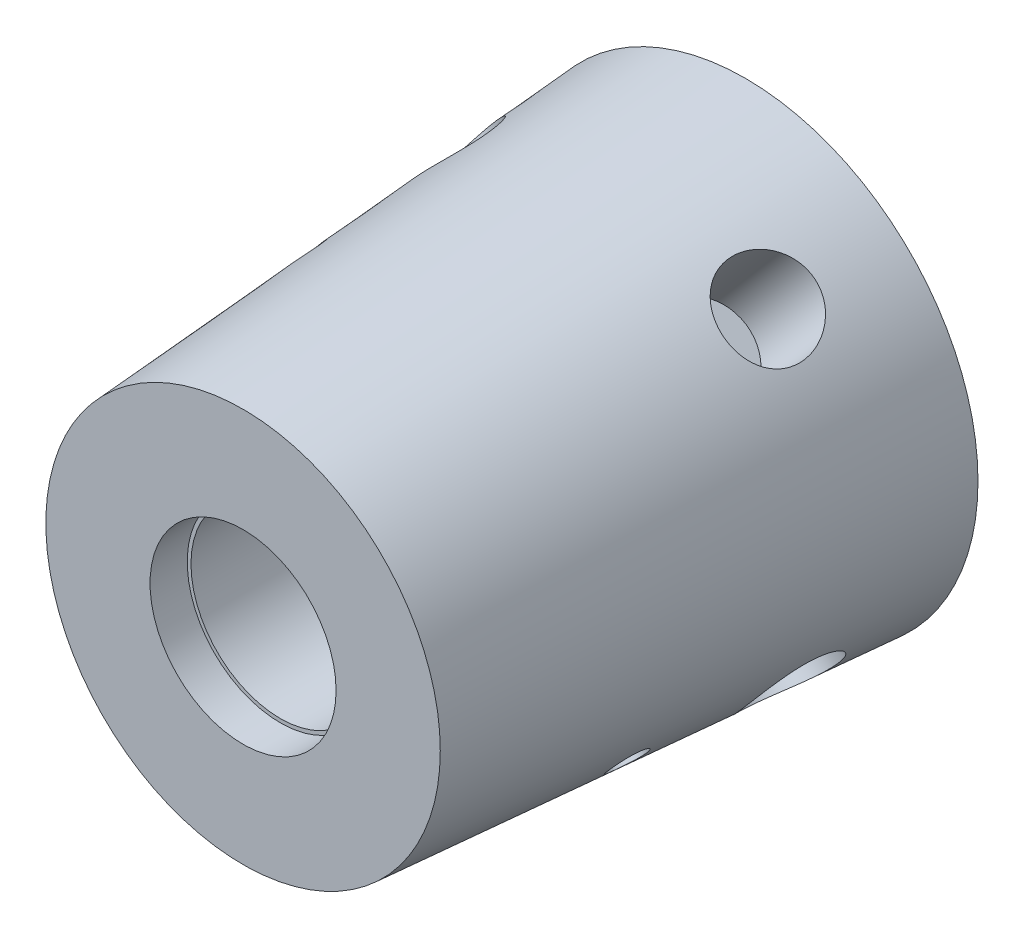
SolidWorks part; units mm, degrees
ref_plane "Front Plane" through (0, 0, 0) normal (0, 0, 1) x (1, 0, 0)
ref_plane "Top Plane" through (0, 0, 0) normal (0, 1, 0) x (1, 0, 0)
ref_plane "Right Plane" through (0, 0, 0) normal (1, 0, 0) x (0, 0, -1)
ref_plane "Plane1" through (0, 234.744, 0) normal (0, 1, 0) x (1, 0, 0)
sketch "Sketch1" plane through (0, 234.744, 0) normal (0, 1, 0) x (1, 0, 0)
  line L0 (583.7306, 1284.9984) -> (521.2306, 1284.9984)
  line L1 (521.2306, 1284.9984) -> (521.2306, 1149.9984)
  line L2 (521.2306, 1149.9984) -> (574.2306, 1149.9984)
  line L3 (574.2306, 1149.9984) -> (583.7306, 1284.9984)
  line L4 (521.2306, 1284.9984) -> (521.2306, 1149.9984) construction
  dimension "D1" = 53
  dimension "D2" = 62.5
  dimension "D3" = 135
revolve "Revolve1" add sketch "Sketch1" angle 360 about L4
ref_plane "Plane2" through (137.8305, -119.5183, 0) normal (-0.7555, 0.6551, 0) x (0, 0, 1)
hole_wizard "Ø10.0 (10) diameter hole1" positions "Sketch3" profile "Sketch2" hole size "Ø10.0" standard "ANSI Metric"
sketch "Sketch3" plane through (137.8305, -119.5183, 0) normal (-0.7555, 0.6551, 0) x (0, 0, 1)
  point P0 (-1209.9984, 518.8281)
sketch "Sketch2" plane through (477.7327, 272.4627, -1209.9984) normal (0, 0, 1) x (-0.6551, -0.7555, 0)
  line L0 (0, 0) -> (0, 22.5741)
  line L1 (0, 22.5741) -> (5, 22.5741)
  line L2 (5, 22.5741) -> (5, 0)
  line L5 (5, 0) -> (0, 0)
  line L10 (0, 22.5741) -> (-5, 22.5741) construction
  line L11 (0, -6.35) -> (0, 107.95) construction
  dimension "孔直径" = 10
  dimension "孔深度" = 22.5741
  dimension "导头角度" = 180
ref_plane "Plane3" through (224.8264, -194.9558, 0) normal (0.7555, -0.6551, 0) x (0, 0, -1)
hole_wizard "Ø10.0 (10) diameter hole2" positions "Sketch5" profile "Sketch4" hole size "Ø10.0" standard "ANSI Metric"
sketch "Sketch5" plane through (224.8264, -194.9558, 0) normal (0.7555, -0.6551, 0) x (0, 0, -1)
  point P0 (1209.9984, 518.8281)
sketch "Sketch4" plane through (564.7286, 197.0252, -1209.9984) normal (0, 0, 1) x (0.6551, 0.7555, 0)
  line L0 (0, 0) -> (0, 22.5741)
  line L1 (0, 22.5741) -> (5, 22.5741)
  line L2 (5, 22.5741) -> (5, 0)
  line L5 (5, 0) -> (0, 0)
  line L10 (0, 22.5741) -> (-5, 22.5741) construction
  line L11 (0, -6.35) -> (0, 107.95) construction
  dimension "孔直径" = 10
  dimension "孔深度" = 22.5741
  dimension "导头角度" = 180
ref_plane "Plane4" through (135.232, -117.265, 0) normal (-0.7555, 0.6551, 0) x (0, 0, 1)
hole_wizard "Ø24.0 (24) diameter hole1" positions "Sketch7" profile "Sketch6" hole size "Ø24.0" standard "ANSI Metric"
sketch "Sketch7" plane through (135.232, -117.265, 0) normal (-0.7555, 0.6551, 0) x (0, 0, 1)
  point P0 (-1251.8739, 518.8281)
sketch "Sketch6" plane through (475.1342, 274.716, -1251.8739) normal (0, 0, 1) x (-0.6551, -0.7555, 0)
  line L0 (0, 0) -> (0, 27.0135)
  line L1 (0, 27.0135) -> (12, 27.0135)
  line L2 (12, 27.0135) -> (12, 0)
  line L5 (12, 0) -> (0, 0)
  line L10 (0, 27.0135) -> (-12, 27.0135) construction
  line L11 (0, -6.35) -> (0, 107.95) construction
  dimension "孔直径" = 24
  dimension "孔深度" = 27.0135
  dimension "导头角度" = 180
ref_plane "Plane5" through (299.9302, 345.8846, 0) normal (-0.6551, -0.7555, 0) x (-0.7555, 0.6551, 0)
hole_wizard "Ø24.0 (24) diameter hole2" positions "Sketch9" profile "Sketch8" hole size "Ø24.0" standard "ANSI Metric"
sketch "Sketch9" plane through (299.9302, 345.8846, 0) normal (-0.6551, -0.7555, 0) x (-0.7555, 0.6551, 0)
  point P0 (-240.0073, 1251.8739)
sketch "Sketch8" plane through (481.2586, 188.6475, -1251.8739) normal (0, 0, 1) x (0.7555, -0.6551, 0)
  line L0 (0, 0) -> (0, 27.0135)
  line L1 (0, 27.0135) -> (12, 27.0135)
  line L2 (12, 27.0135) -> (12, 0)
  line L5 (12, 0) -> (0, 0)
  line L10 (0, 27.0135) -> (-12, 27.0135) construction
  line L11 (0, -6.35) -> (0, 107.95) construction
  dimension "孔直径" = 24
  dimension "孔深度" = 27.0135
  dimension "导头角度" = 180
ref_plane "Plane6" through (379.8742, 438.0774, 0) normal (0.6551, 0.7555, 0) x (0.7555, -0.6551, 0)
hole_wizard "Ø24.0 (24) diameter hole3" positions "Sketch11" profile "Sketch10" hole size "Ø24.0" standard "ANSI Metric"
sketch "Sketch11" plane through (379.8742, 438.0774, 0) normal (0.6551, 0.7555, 0) x (0.7555, -0.6551, 0)
  point P0 (240.0073, 1251.8739)
sketch "Sketch10" plane through (561.2027, 280.8404, -1251.8739) normal (0, 0, 1) x (-0.7555, 0.6551, 0)
  line L0 (0, 0) -> (0, 27.0135)
  line L1 (0, 27.0135) -> (12, 27.0135)
  line L2 (12, 27.0135) -> (12, 0)
  line L5 (12, 0) -> (0, 0)
  line L10 (0, 27.0135) -> (-12, 27.0135) construction
  line L11 (0, -6.35) -> (0, 107.95) construction
  dimension "孔直径" = 24
  dimension "孔深度" = 27.0135
  dimension "导头角度" = 180
ref_plane "Plane7" through (227.4249, -197.2091, 0) normal (0.7555, -0.6551, 0) x (0, 0, -1)
hole_wizard "Ø24.0 (24) diameter hole4" positions "Sketch13" profile "Sketch12" hole size "Ø24.0" standard "ANSI Metric"
sketch "Sketch13" plane through (227.4249, -197.2091, 0) normal (0.7555, -0.6551, 0) x (0, 0, -1)
  point P0 (1251.8739, 518.8281)
sketch "Sketch12" plane through (567.3271, 194.7719, -1251.8739) normal (0, 0, 1) x (0.6551, 0.7555, 0)
  line L0 (0, 0) -> (0, 27.0135)
  line L1 (0, 27.0135) -> (12, 27.0135)
  line L2 (12, 27.0135) -> (12, 0)
  line L5 (12, 0) -> (0, 0)
  line L10 (0, 27.0135) -> (-12, 27.0135) construction
  line L11 (0, -6.35) -> (0, 107.95) construction
  dimension "孔直径" = 24
  dimension "孔深度" = 27.0135
  dimension "导头角度" = 180
hole_wizard "M42 counterbore hole1" positions "Sketch15" profile "Sketch14" counterbore size "M42" standard "ANSI Metric"
sketch "Sketch15" plane through (0, 0, -1149.9984) normal (0, 0, 1) x (1, 0, 0)
  point P0 (521.2306, 234.744)
sketch "Sketch14" plane through (521.2306, 234.744, -1149.9984) normal (1, 0, 0) x (0, -1, 0)
  line L0 (0, 0) -> (0, 135)
  line L1 (0, 135) -> (24, 135)
  line L3 (24, 135) -> (24, 10)
  line L4 (24, 10) -> (25, 10)
  line L5 (25, 10) -> (25, 0)
  line L7 (25, 0) -> (0, 0)
  line L11 (0, -6.35) -> (0, 107.95) construction
  dimension "通孔孔直径" = 48
  dimension "通孔孔深度" = 135
  dimension "柱形沉头孔直径" = 50
  dimension "柱形沉头孔深度" = 10
